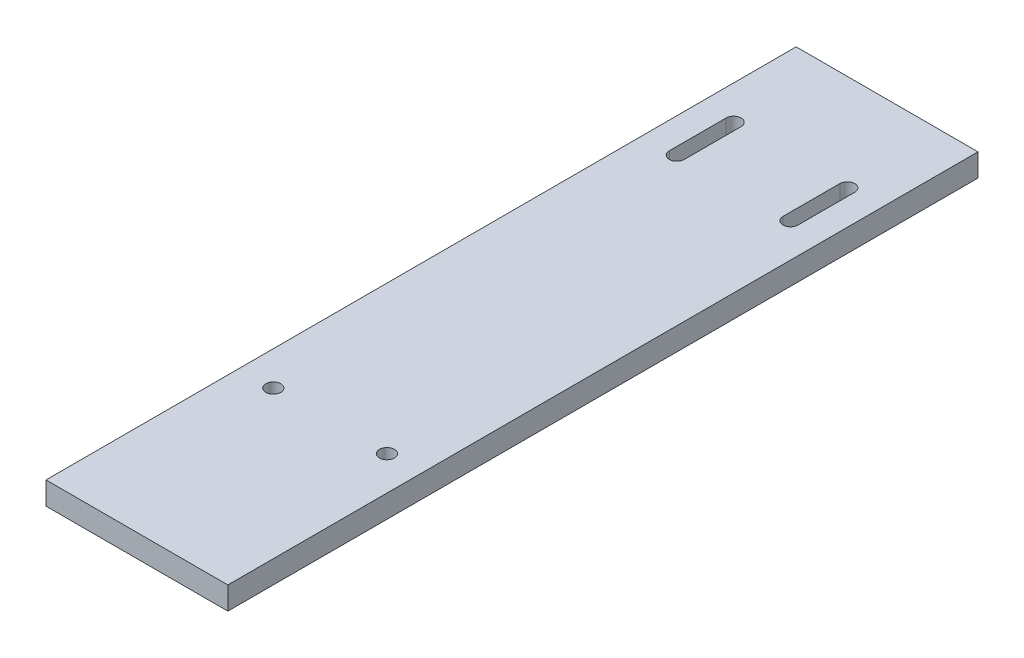
SolidWorks part; units mm, degrees
ref_plane "Front Plane" through (0, 0, 0) normal (0, 0, 1) x (1, 0, 0)
ref_plane "Top Plane" through (0, 0, 0) normal (0, 1, 0) x (1, 0, 0)
ref_plane "Right Plane" through (0, 0, 0) normal (1, 0, 0) x (0, 0, -1)
sketch "Sketch1" plane through (0, 0, 0) normal (0, 1, 0) x (1, 0, 0)
  line L1 (-40, 165) -> (40, 165)
  line L2 (-40, 165) -> (-40, -165)
  line L3 (-40, -165) -> (40, -165)
  line L4 (40, 165) -> (40, -165)
  line L5 (-40, 165) -> (40, -165) construction
  line L6 (-40, -165) -> (40, 165) construction
  point P0 (0, 0)
  dimension "D1" = 330
  dimension "D2" = 80
extrude "Boss-Extrude1" add sketch "Sketch1" along normal blind 10
sketch "Sketch2" plane through (0, 10, 0) normal (0, 1, 0) x (1, 0, 0)
  line L0 (0, 0) -> (0, 15) construction
  line L1 (-25, 110) -> (25, 110) construction
  line L2 (-25, 110) -> (-25, -80) construction
  line L3 (-25, -80) -> (25, -80) construction
  line L4 (25, 110) -> (25, -80) construction
  line L5 (-25, 110) -> (25, -80) construction
  line L6 (-25, -80) -> (25, 110) construction
  point P0 (0, 15)
  dimension "D1" = 50
  dimension "D2" = 190
  dimension "D3" = 80
hole_wizard "Ø6.6 (6.6) Diameter Hole1" positions "Sketch3" profile "Sketch4" hole size "Ø6.6" standard "GB" end condition up to next
sketch "Sketch3" plane through (0, 10, 0) normal (0, 1, 0) x (1, 0, 0)
  point P6 (-25, -80)
  point P9 (25, -80)
sketch "Sketch4" plane through (-25, 10, 80) normal (1, 0, 0) x (0, 0, 1)
  line L0 (0, 0) -> (0, 10)
  line L1 (0, 10) -> (3.3, 10)
  line L2 (3.3, 10) -> (3.3, 0)
  line L5 (3.3, 0) -> (0, 0)
  line L11 (0, -6.35) -> (0, 107.95) construction
  dimension "通孔孔直径" = 6.6
  dimension "通孔孔深度" = 10
sketch "Sketch5" plane through (0, 10, 0) normal (0, 1, 0) x (1, 0, 0)
  line L0 (-25, 97.5) -> (-25, 122.5) construction
  line L1 (-28.3, 97.5) -> (-28.3, 122.5)
  line L2 (-21.7, 97.5) -> (-21.7, 122.5)
  line L3 (25, 97.5) -> (25, 122.5) construction
  line L4 (21.7, 97.5) -> (21.7, 122.5)
  line L5 (28.3, 97.5) -> (28.3, 122.5)
  arc A0 (-28.3, 97.5) -> (-21.7, 97.5) centre (-25, 97.5) ccw
  arc A1 (-21.7, 122.5) -> (-28.3, 122.5) centre (-25, 122.5) ccw
  arc A2 (21.7, 97.5) -> (28.3, 97.5) centre (25, 97.5) ccw
  arc A3 (28.3, 122.5) -> (21.7, 122.5) centre (25, 122.5) ccw
  point P2 (-25, 110)
  point P9 (25, 110)
  dimension "D1" = 3.3
  dimension "D2" = 3.3
  dimension "D3" = 25
  dimension "D4" = 25
extrude "Cut-Extrude1" cut sketch "Sketch5" against normal blind 10
